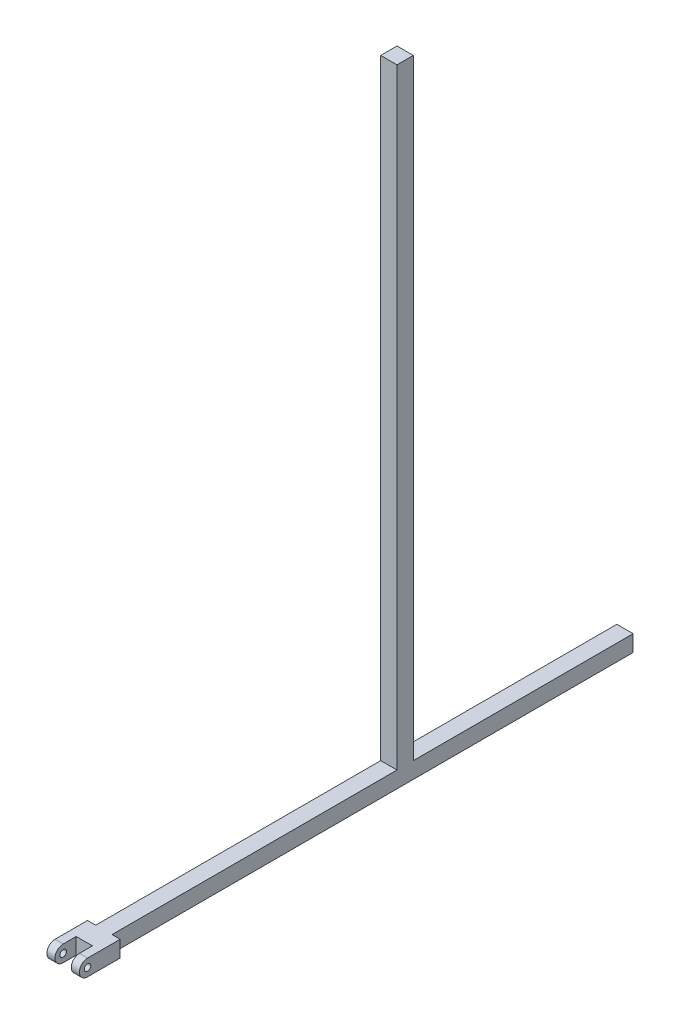
from build123d import *

# Parameters (mm, degrees)
SKETCH1_W               = 5
SKETCH1_H               = 5
BOSS_EXTRUDE1_DEPTH     = 160
SKETCH2_W               = 10
SKETCH2_H               = 5
BOSS_EXTRUDE2_DEPTH     = 18
SKETCH3_W               = 5
SKETCH3_H               = 19.358131828
CUT_EXTRUDE1_DEPTH      = 12
CUT_EXTRUDE2_DEPTH      = 179.298205263
CUT_EXTRUDE2_DEPTH_BACK = 179.298205263
SKETCH4_R               = 1
SKETCH5_W               = 5
SKETCH5_H               = 5
BOSS_EXTRUDE3_DEPTH     = 190


with BuildPart() as part:
    # Sketch1 → Boss-Extrude1 (new body)
    with BuildSketch(Plane.XY):
        Rectangle(SKETCH1_W, SKETCH1_H)
    extrude(amount=BOSS_EXTRUDE1_DEPTH)

    # Sketch2 → Boss-Extrude2 (add)
    with BuildSketch(Plane.XY.offset(160)):
        Rectangle(SKETCH2_W, SKETCH2_H)
    extrude(amount=BOSS_EXTRUDE2_DEPTH)

    # Sketch3 → Cut-Extrude1 (cut)
    with BuildSketch(Plane.XY.offset(178)):
        Rectangle(SKETCH3_W, SKETCH3_H)
    extrude(amount=-CUT_EXTRUDE1_DEPTH, mode=Mode.SUBTRACT)

    # Sketch4 → Cut-Extrude2 (cut, two sides: drawn at the far end of the back side and taken through both)
    with BuildSketch(Plane(origin=(5, 0, 0), x_dir=(0, 0, -1), z_dir=(1, 0, 0)).offset(-CUT_EXTRUDE2_DEPTH_BACK)):
        with Locations(Location((-170, 0, 0), (0, 0, 90))):
            Circle(SKETCH4_R)
        with BuildLine():
            Line((-170, 2.5), (-170, 12.575428257))
            Line((-170, 12.575428257), (-197.273990227, 12.575428257))
            Line((-197.273990227, 12.575428257), (-202.218051786, -13.998902623))
            Line((-202.218051786, -13.998902623), (-170, -2.5))
            ThreePointArc((-170, -2.5), (-172.5, 0), (-170, 2.5))
        make_face()
    extrude(amount=CUT_EXTRUDE2_DEPTH + CUT_EXTRUDE2_DEPTH_BACK, mode=Mode.SUBTRACT)

    # Sketch5 → Boss-Extrude3 (add)
    with BuildSketch(Plane(origin=(0, 0, 0), x_dir=(1, 0, 0), z_dir=(0, 1, 0))):
        with Locations((0, -70)):
            Rectangle(SKETCH5_W, SKETCH5_H)
    extrude(amount=BOSS_EXTRUDE3_DEPTH)


solid = part.part
